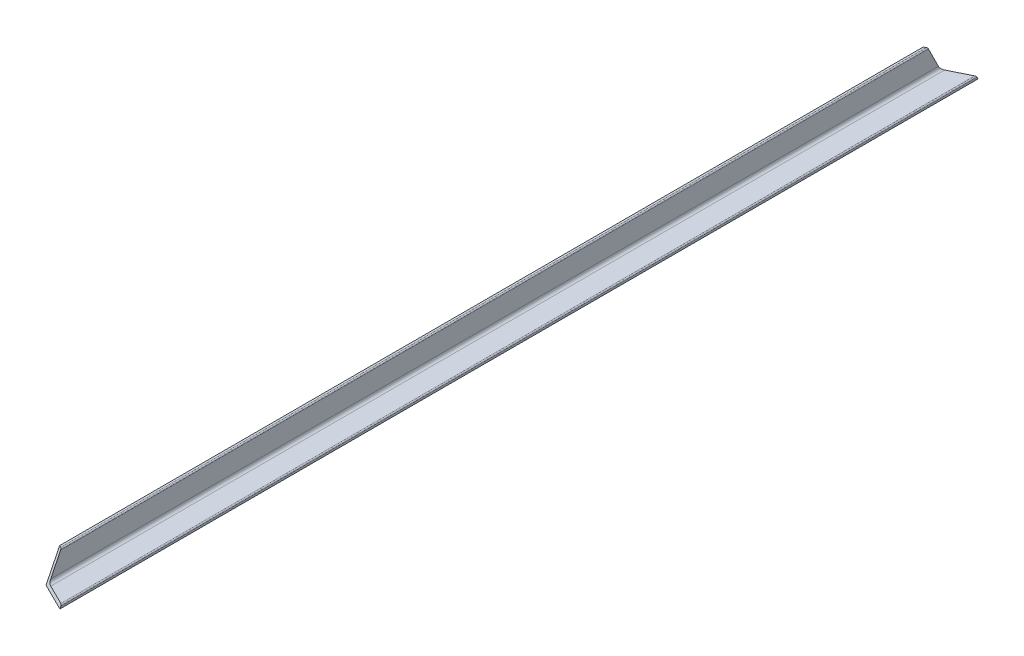
from build123d import *

# Parameters (mm, degrees)
BOSS_EXTRUDE1_DEPTH     = 2334
CUT_EXTRUDE4_DEPTH      = 2337.098456829
CUT_EXTRUDE4_DEPTH_BACK = 10


with BuildPart() as part:
    # Sketch1 → Boss-Extrude1 (new body)
    with BuildSketch(Plane.XY):
        with BuildLine():
            Line((0, 70), (0, 0))
            Line((0, 0), (70, 0))
            Line((70, 0), (70, 5))
            ThreePointArc((70, 5), (69.121320344, 7.121320344), (67, 8))
            Line((67, 8), (16, 8))
            ThreePointArc((16, 8), (10.343145751, 10.343145751), (8, 16))
            Line((8, 16), (8, 67))
            ThreePointArc((8, 67), (7.121320344, 69.121320344), (5, 70))
            Line((5, 70), (0, 70))
        make_face()
    extrude(amount=BOSS_EXTRUDE1_DEPTH)

    # Sketch3 → Cut-Extrude4 (cut, two sides: drawn at the far end of the back side and taken through both)
    with BuildSketch(Plane(origin=(0, 0, 0), x_dir=(0, 0, -1), z_dir=(0.7071067811865488, 0.7071067811865464, 0)).offset(-CUT_EXTRUDE4_DEPTH_BACK)):
        Polygon((0, -49.497474683), (-69.317009791, 49.497474683), (0, 49.497474683), align=None)
        Polygon((-2334, -49.497474683), (-2334, 49.497474683), (-2264.682990209, 49.497474683), align=None)
    extrude(amount=CUT_EXTRUDE4_DEPTH + CUT_EXTRUDE4_DEPTH_BACK, mode=Mode.SUBTRACT)


solid = part.part
